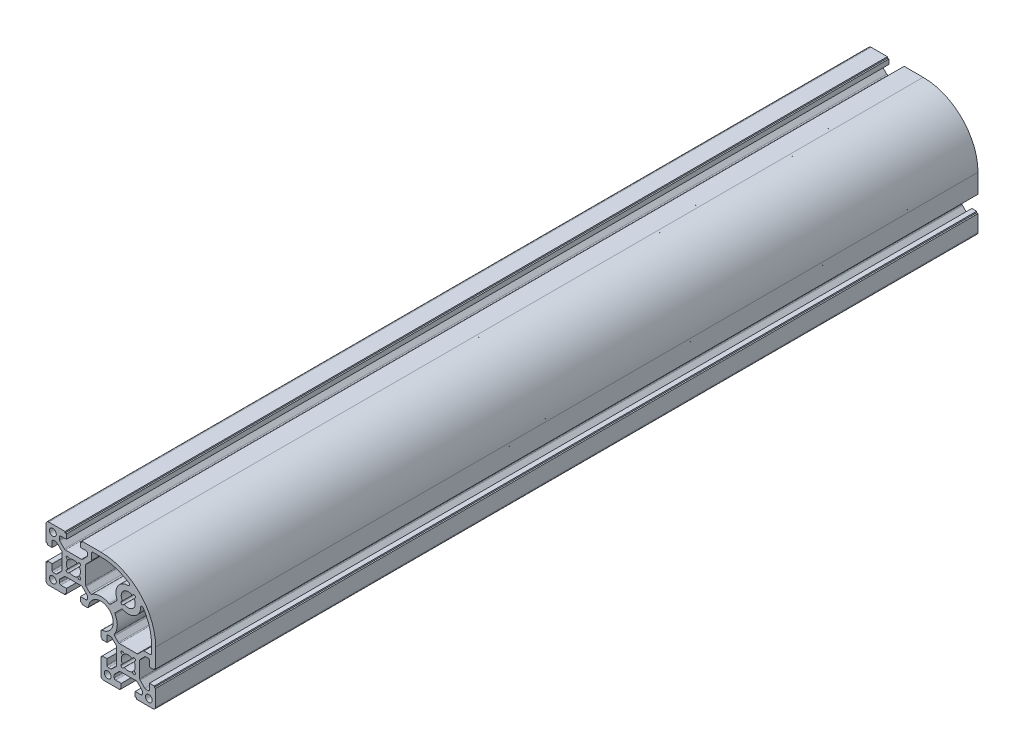
SolidWorks part; units mm, degrees
ref_plane "Front Plane" through (0, 0, 0) normal (0, 0, 1) x (1, 0, 0)
ref_plane "Top Plane" through (0, 0, 0) normal (0, 1, 0) x (1, 0, 0)
ref_plane "Right Plane" through (0, 0, 0) normal (1, 0, 0) x (0, 0, -1)
sketch "Sketch1" plane through (0, 0, 0) normal (0, 0, 1) x (1, 0, 0)
  line L0 (-23.6087, 14.979) -> (-22.8307, 15.757)
  line L1 (-17.1727, 15.757) -> (-16.3944, 14.9787)
  line L2 (-14.9799, 16.3932) -> (-15.7577, 17.171)
  line L3 (-15.7577, 22.829) -> (-14.9799, 23.6067)
  line L4 (-16.3943, 25.0214) -> (-17.1727, 24.244)
  line L5 (-22.8307, 24.244) -> (-23.6087, 25.021)
  line L6 (-25.0227, 23.607) -> (-24.2447, 22.829)
  line L7 (-24.2447, 17.171) -> (-25.0227, 16.393)
  line L8 (27.1702, -10.7071) -> (30.8344, -7.0429)
  line L9 (31.5415, -6.75) -> (35.9983, -6.75)
  line L10 (36.9983, -5.75) -> (36.9983, 0.0007)
  line L11 (15.0925, 11.5582) -> (10.6198, 7.0854)
  line L12 (10.0802, -7.9599) -> (12.8274, -10.7071)
  line L13 (13.5345, -11) -> (26.4631, -11)
  line L14 (7.0844, 10.6211) -> (11.56, 15.0967)
  line L15 (0, 37) -> (-5.7517, 37)
  line L16 (-6.7517, 36) -> (-6.7517, 31.5432)
  line L17 (-7.0446, 30.8361) -> (-10.7088, 27.1719)
  line L18 (-11.0017, 26.4648) -> (-11.0017, 13.5362)
  line L19 (-10.7088, 12.8291) -> (-7.9615, 10.0819)
  line L20 (23.5883, 24.909) -> (22.8103, 24.131)
  line L21 (15.7383, 17.059) -> (14.9601, 16.2807)
  line L22 (16.3746, 14.8662) -> (17.1523, 15.644)
  line L23 (24.2243, 22.717) -> (25.0023, 23.495)
  line L24 (16.3913, -25.021) -> (17.1693, -24.243)
  line L25 (22.8273, -24.243) -> (23.6056, -25.0213)
  line L26 (25.0201, -23.6068) -> (24.2423, -22.829)
  line L27 (24.2423, -17.171) -> (25.0201, -16.3933)
  line L28 (23.6057, -14.9786) -> (22.8273, -15.756)
  line L29 (17.1693, -15.756) -> (16.3913, -14.979)
  line L30 (14.9773, -16.393) -> (15.7553, -17.171)
  line L31 (15.7553, -22.829) -> (14.9773, -23.607)
  line L32 (-25.1017, 35.5) -> (-25.1017, 39)
  line L33 (-29.2517, 35.5) -> (-25.1017, 35.5)
  line L34 (-30.2517, 32.7862) -> (-30.2517, 34.5)
  line L35 (-26.5726, 28.6929) -> (-29.9588, 32.0791)
  line L36 (-14.1369, 28.4) -> (-25.8655, 28.4)
  line L37 (-10.0445, 32.0792) -> (-13.4297, 28.693)
  line L38 (-9.7517, 34.5) -> (-9.7517, 32.7862)
  line L39 (-14.9017, 35.5) -> (-10.7517, 35.5)
  line L40 (-14.9017, 39) -> (-14.9017, 35.5)
  line L41 (-13.9017, 39) -> (-14.9017, 39)
  line L42 (-13.9017, 40) -> (-13.9017, 39)
  line L43 (-0.0017, 40) -> (-13.9017, 40)
  line L44 (39.9983, -13.9) -> (39.9983, 0)
  line L45 (38.9983, -13.9) -> (39.9983, -13.9)
  line L46 (38.9983, -14.9) -> (38.9983, -13.9)
  line L47 (35.4983, -14.9) -> (38.9983, -14.9)
  line L48 (35.4983, -10.75) -> (35.4983, -14.9)
  line L49 (32.7845, -9.75) -> (34.4983, -9.75)
  line L50 (28.6913, -13.428) -> (32.0775, -10.0428)
  line L51 (28.3983, -25.8638) -> (28.3983, -14.1352)
  line L52 (32.0774, -29.9571) -> (28.6912, -26.5709)
  line L53 (34.4983, -30.25) -> (32.7845, -30.25)
  line L54 (35.4983, -25.1) -> (35.4983, -29.25)
  line L55 (38.9983, -25.1) -> (35.4983, -25.1)
  line L56 (38.9983, -26.1) -> (38.9983, -25.1)
  line L57 (39.9983, -26.1) -> (38.9983, -26.1)
  line L58 (39.9983, -38) -> (39.9983, -26.1)
  line L59 (26.0983, -40) -> (37.9983, -40)
  line L60 (26.0983, -39) -> (26.0983, -40)
  line L61 (25.0983, -39) -> (26.0983, -39)
  line L62 (25.0983, -35.5) -> (25.0983, -39)
  line L63 (29.2483, -35.5) -> (25.0983, -35.5)
  line L64 (30.2483, -32.7852) -> (30.2483, -34.5)
  line L65 (26.5702, -28.6929) -> (29.9554, -32.0781)
  line L66 (14.1345, -28.4) -> (25.8631, -28.4)
  line L67 (10.0413, -32.078) -> (13.4275, -28.6928)
  line L68 (9.7483, -34.5) -> (9.7483, -32.7852)
  line L69 (14.8983, -35.5) -> (10.7483, -35.5)
  line L70 (14.8983, -39) -> (14.8983, -35.5)
  line L71 (13.8983, -39) -> (14.8983, -39)
  line L72 (13.8983, -40) -> (13.8983, -39)
  line L73 (1.9983, -40) -> (13.8983, -40)
  line L74 (-0.0017, -26.1) -> (-0.0017, -38)
  line L75 (0.9983, -26.1) -> (-0.0017, -26.1)
  line L76 (0.9983, -25.1) -> (0.9983, -26.1)
  line L77 (4.4983, -25.1) -> (0.9983, -25.1)
  line L78 (4.4983, -29.25) -> (4.4983, -25.1)
  line L79 (7.2131, -30.25) -> (5.4983, -30.25)
  line L80 (11.3055, -26.5708) -> (7.9203, -29.957)
  line L81 (11.5983, -14.1352) -> (11.5983, -25.8638)
  line L82 (7.9202, -10.0429) -> (11.3054, -13.4281)
  line L83 (5.4983, -9.75) -> (7.2131, -9.75)
  line L84 (4.4983, -14.9) -> (4.4983, -10.75)
  line L85 (0.9983, -14.9) -> (4.4983, -14.9)
  line L86 (0.9983, -13.9) -> (0.9983, -14.9)
  line L87 (-0.0017, -13.9) -> (0.9983, -13.9)
  line L88 (-0.0017, -9.95) -> (-0.0017, -13.9)
  line L89 (-13.9017, 0) -> (-9.9517, 0)
  line L90 (-13.9017, 1) -> (-13.9017, 0)
  line L91 (-14.9017, 1) -> (-13.9017, 1)
  line L92 (-14.9017, 4.5) -> (-14.9017, 1)
  line L93 (-10.7517, 4.5) -> (-14.9017, 4.5)
  line L94 (-9.7517, 7.2148) -> (-9.7517, 5.5)
  line L95 (-13.4298, 11.3071) -> (-10.0446, 7.9219)
  line L96 (-25.8655, 11.6) -> (-14.1369, 11.6)
  line L97 (-29.9587, 7.922) -> (-26.5725, 11.3072)
  line L98 (-30.2517, 5.5) -> (-30.2517, 7.2148)
  line L99 (-25.1017, 4.5) -> (-29.2517, 4.5)
  line L100 (-25.1017, 1) -> (-25.1017, 4.5)
  line L101 (-26.1017, 1) -> (-25.1017, 1)
  line L102 (-26.1017, 0) -> (-26.1017, 1)
  line L103 (-38.0017, 0) -> (-26.1017, 0)
  line L104 (-40.0017, 13.9) -> (-40.0017, 2)
  line L105 (-39.0017, 13.9) -> (-40.0017, 13.9)
  line L106 (-39.0017, 14.9) -> (-39.0017, 13.9)
  line L107 (-35.5017, 14.9) -> (-39.0017, 14.9)
  line L108 (-35.5017, 10.75) -> (-35.5017, 14.9)
  line L109 (-32.7869, 9.75) -> (-34.5017, 9.75)
  line L110 (-28.6945, 13.4292) -> (-32.0797, 10.043)
  line L111 (-28.4017, 25.8648) -> (-28.4017, 14.1362)
  line L112 (-32.0798, 29.9571) -> (-28.6946, 26.5719)
  line L113 (-34.5017, 30.25) -> (-32.7869, 30.25)
  line L114 (-35.5017, 25.1) -> (-35.5017, 29.25)
  line L115 (-39.0017, 25.1) -> (-35.5017, 25.1)
  line L116 (-39.0017, 26.1) -> (-39.0017, 25.1)
  line L117 (-40.0017, 26.1) -> (-39.0017, 26.1)
  line L118 (-40.0017, 38) -> (-40.0017, 26.1)
  line L119 (-26.1017, 40) -> (-38.0017, 40)
  line L120 (-26.1017, 39) -> (-26.1017, 40)
  line L121 (-25.1017, 39) -> (-26.1017, 39)
  circle A0 centre (-35.0017, 35) radius 2.5
  arc A1 (-25.0227, 16.393) -> (-23.6087, 14.979) centre (-24.3034, 15.6983) ccw
  arc A2 (-22.8307, 15.757) -> (-17.1727, 15.757) centre (-20.0017, 20.0004) ccw
  arc A3 (-16.3944, 14.9787) -> (-14.9799, 16.3932) centre (-15.6872, 15.686) ccw
  arc A4 (-15.7577, 17.171) -> (-15.7577, 22.829) centre (-20.0011, 20) ccw
  arc A5 (-14.9799, 23.6067) -> (-16.3943, 25.0214) centre (-15.6875, 24.3137) ccw
  arc A6 (-17.1727, 24.244) -> (-22.8307, 24.244) centre (-20.0017, 20.0006) ccw
  arc A7 (-23.6087, 25.021) -> (-25.0227, 23.607) centre (-24.3034, 24.3017) ccw
  arc A8 (-24.2447, 22.829) -> (-24.2447, 17.171) centre (-20.0012, 20) ccw
  arc A9 (26.4631, -11) -> (27.1702, -10.7071) centre (26.4631, -10) ccw
  arc A10 (31.5415, -6.75) -> (30.8344, -7.0429) centre (31.5415, -7.75) ccw
  arc A11 (35.9983, -6.75) -> (36.9983, -5.75) centre (35.9983, -5.75) ccw
  arc A12 (36.9983, 0.0007) -> (30.9163, 20.325) centre (-0.0017, 0.0007) ccw
  arc A13 (30.9163, 20.325) -> (29.0803, 19.787) centre (30.0803, 19.7764) ccw
  arc A14 (16.2273, 11.755) -> (29.0803, 19.787) centre (20.0809, 19.8883) ccw
  arc A15 (16.2273, 11.755) -> (15.0925, 11.5582) centre (15.7996, 10.8511) ccw
  arc A16 (10.6198, 7.0854) -> (10.4553, 5.888) centre (11.3269, 6.3783) ccw
  arc A17 (9.9573, -6.695) -> (10.4553, 5.888) centre (-0.0011, 0.0005) ccw
  arc A18 (9.9573, -6.695) -> (10.0802, -7.9599) centre (10.7873, -7.2528) ccw
  arc A19 (12.8274, -10.7071) -> (13.5345, -11) centre (13.5345, -10) ccw
  arc A20 (-7.9615, 10.0819) -> (-6.6967, 9.959) centre (-7.2544, 10.789) ccw
  arc A21 (5.8863, 10.457) -> (-6.6967, 9.959) centre (-0.0012, 0.0006) ccw
  arc A22 (5.8863, 10.457) -> (7.0844, 10.6211) centre (6.3773, 11.3282) ccw
  arc A23 (11.56, 15.0967) -> (11.7653, 16.213) centre (10.8529, 15.8038) ccw
  arc A24 (20.0593, 28.887) -> (11.7653, 16.213) centre (19.9811, 19.8873) ccw
  arc A25 (20.0593, 28.887) -> (20.6253, 30.718) centre (20.0691, 29.887) ccw
  arc A26 (20.6253, 30.718) -> (0, 37) centre (0, 0) ccw
  arc A27 (-5.7517, 37) -> (-6.7517, 36) centre (-5.7517, 36) ccw
  arc A28 (-7.0446, 30.8361) -> (-6.7517, 31.5432) centre (-7.7517, 31.5432) ccw
  arc A29 (-10.7088, 27.1719) -> (-11.0017, 26.4648) centre (-10.0017, 26.4648) ccw
  arc A30 (-11.0017, 13.5362) -> (-10.7088, 12.8291) centre (-10.0017, 13.5362) ccw
  arc A31 (25.0023, 23.495) -> (23.5883, 24.909) centre (24.283, 24.1897) ccw
  arc A32 (22.8103, 24.131) -> (15.7383, 17.059) centre (19.9826, 19.8867) ccw
  arc A33 (14.9601, 16.2807) -> (16.3746, 14.8662) centre (15.6673, 15.5735) ccw
  arc A34 (17.1523, 15.644) -> (24.2243, 22.717) centre (19.9812, 19.8875) ccw
  circle A35 centre (4.9983, -35) radius 2.5
  arc A36 (14.9773, -23.607) -> (16.3913, -25.021) centre (15.6966, -24.3017) ccw
  arc A37 (17.1693, -24.243) -> (22.8273, -24.243) centre (19.9983, -19.9996) ccw
  arc A38 (23.6056, -25.0213) -> (25.0201, -23.6068) centre (24.3128, -24.314) ccw
  arc A39 (24.2423, -22.829) -> (24.2423, -17.171) centre (19.9989, -20) ccw
  arc A40 (25.0201, -16.3933) -> (23.6057, -14.9786) centre (24.3125, -15.6863) ccw
  arc A41 (22.8273, -15.756) -> (17.1693, -15.756) centre (19.9983, -19.9994) ccw
  arc A42 (16.3913, -14.979) -> (14.9773, -16.393) centre (15.6966, -15.6983) ccw
  arc A43 (15.7553, -17.171) -> (15.7553, -22.829) centre (19.9988, -20) ccw
  arc A44 (-29.2517, 35.5) -> (-30.2517, 34.5) centre (-29.2517, 34.5) ccw
  arc A45 (-30.2517, 32.7862) -> (-29.9588, 32.0791) centre (-29.2517, 32.7862) ccw
  arc A46 (-26.5726, 28.6929) -> (-25.8655, 28.4) centre (-25.8655, 29.4) ccw
  arc A47 (-14.1369, 28.4) -> (-13.4297, 28.693) centre (-14.1369, 29.4) ccw
  arc A48 (-10.0445, 32.0792) -> (-9.7517, 32.7862) centre (-10.7517, 32.7862) ccw
  arc A49 (-9.7517, 34.5) -> (-10.7517, 35.5) centre (-10.7517, 34.5) ccw
  arc A50 (39.9983, 0) -> (-0.0017, 40) centre (-0.0017, 0) ccw
  arc A51 (35.4983, -10.75) -> (34.4983, -9.75) centre (34.4983, -10.75) ccw
  arc A52 (32.7845, -9.75) -> (32.0775, -10.0428) centre (32.7845, -10.75) ccw
  arc A53 (28.6913, -13.428) -> (28.3983, -14.1352) centre (29.3983, -14.1352) ccw
  arc A54 (28.3983, -25.8638) -> (28.6912, -26.5709) centre (29.3983, -25.8638) ccw
  arc A55 (32.0774, -29.9571) -> (32.7845, -30.25) centre (32.7845, -29.25) ccw
  arc A56 (34.4983, -30.25) -> (35.4983, -29.25) centre (34.4983, -29.25) ccw
  arc A57 (37.9983, -40) -> (39.9983, -38) centre (37.9983, -38) ccw
  arc A58 (29.2483, -35.5) -> (30.2483, -34.5) centre (29.2483, -34.5) ccw
  arc A59 (30.2483, -32.7852) -> (29.9554, -32.0781) centre (29.2483, -32.7852) ccw
  arc A60 (26.5702, -28.6929) -> (25.8631, -28.4) centre (25.8631, -29.4) ccw
  arc A61 (14.1345, -28.4) -> (13.4275, -28.6928) centre (14.1345, -29.4) ccw
  arc A62 (10.0413, -32.078) -> (9.7483, -32.7852) centre (10.7483, -32.7852) ccw
  arc A63 (9.7483, -34.5) -> (10.7483, -35.5) centre (10.7483, -34.5) ccw
  arc A64 (-0.0017, -38) -> (1.9983, -40) centre (1.9983, -38) ccw
  arc A65 (4.4983, -29.25) -> (5.4983, -30.25) centre (5.4983, -29.25) ccw
  arc A66 (7.2131, -30.25) -> (7.9203, -29.957) centre (7.2131, -29.25) ccw
  arc A67 (11.3055, -26.5708) -> (11.5983, -25.8638) centre (10.5983, -25.8638) ccw
  arc A68 (11.5983, -14.1352) -> (11.3054, -13.4281) centre (10.5983, -14.1352) ccw
  arc A69 (7.9202, -10.0429) -> (7.2131, -9.75) centre (7.2131, -10.75) ccw
  arc A70 (5.4983, -9.75) -> (4.4983, -10.75) centre (5.4983, -10.75) ccw
  arc A71 (0.8983, -8.955) -> (-0.0017, -9.95) centre (0.9983, -9.95) ccw
  arc A72 (0.8983, -8.955) -> (-8.9567, 0.9) centre (-0.0018, -0.0001) ccw
  arc A73 (-9.9517, 0) -> (-8.9567, 0.9) centre (-9.9517, 1) ccw
  arc A74 (-10.7517, 4.5) -> (-9.7517, 5.5) centre (-10.7517, 5.5) ccw
  arc A75 (-9.7517, 7.2148) -> (-10.0446, 7.9219) centre (-10.7517, 7.2148) ccw
  arc A76 (-13.4298, 11.3071) -> (-14.1369, 11.6) centre (-14.1369, 10.6) ccw
  arc A77 (-25.8655, 11.6) -> (-26.5725, 11.3072) centre (-25.8655, 10.6) ccw
  arc A78 (-29.9587, 7.922) -> (-30.2517, 7.2148) centre (-29.2517, 7.2148) ccw
  arc A79 (-30.2517, 5.5) -> (-29.2517, 4.5) centre (-29.2517, 5.5) ccw
  arc A80 (-40.0017, 2) -> (-38.0017, 0) centre (-38.0017, 2) ccw
  arc A81 (-35.5017, 10.75) -> (-34.5017, 9.75) centre (-34.5017, 10.75) ccw
  arc A82 (-32.7869, 9.75) -> (-32.0797, 10.043) centre (-32.7869, 10.75) ccw
  arc A83 (-28.6945, 13.4292) -> (-28.4017, 14.1362) centre (-29.4017, 14.1362) ccw
  arc A84 (-28.4017, 25.8648) -> (-28.6946, 26.5719) centre (-29.4017, 25.8648) ccw
  arc A85 (-32.0798, 29.9571) -> (-32.7869, 30.25) centre (-32.7869, 29.25) ccw
  arc A86 (-34.5017, 30.25) -> (-35.5017, 29.25) centre (-34.5017, 29.25) ccw
  arc A87 (-38.0017, 40) -> (-40.0017, 38) centre (-38.0017, 38) ccw
  circle A88 centre (34.9983, -35) radius 2.5
  circle A89 centre (-35.0017, 5) radius 2.5
extrude "Boss-Extrude1" add sketch "Sketch1" along normal mid plane 600
